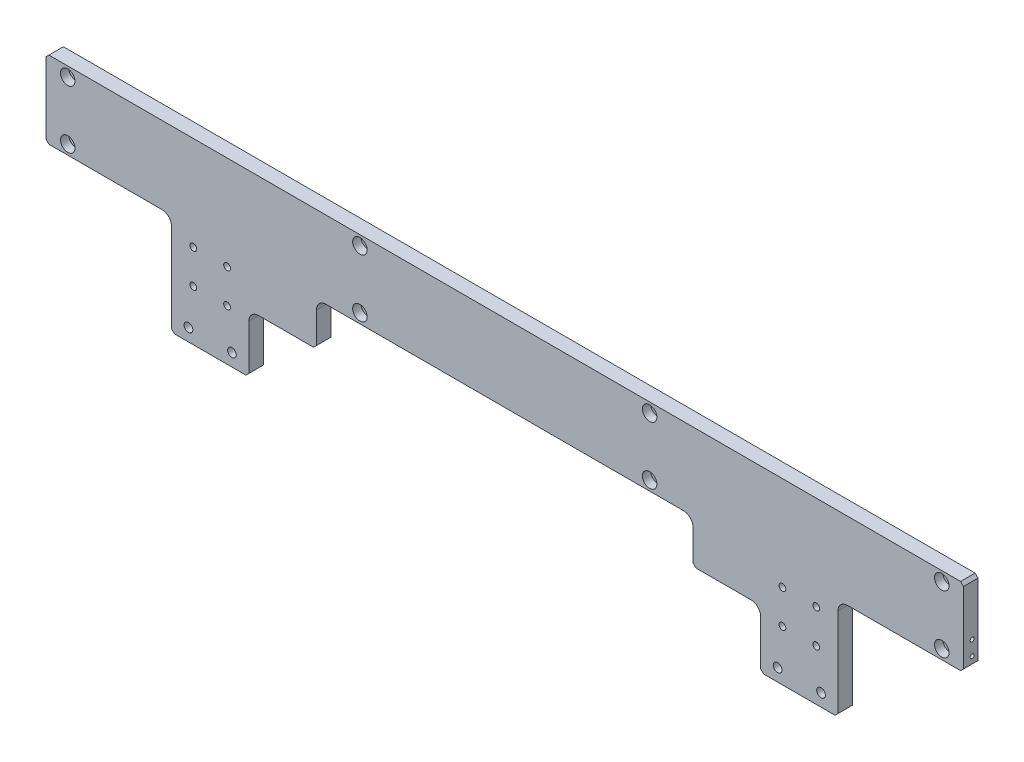
SolidWorks part; units mm, degrees
ref_plane "前视基准面" through (0, 0, 0) normal (0, 0, 1) x (1, 0, 0)
ref_plane "上视基准面" through (0, 0, 0) normal (0, 1, 0) x (1, 0, 0)
ref_plane "右视基准面" through (0, 0, 0) normal (1, 0, 0) x (0, 0, -1)
sketch "草图1" plane through (0, 0, 0) normal (0, 0, 1) x (1, 0, 0)
  line L1 (-475, 40) -> (475, 40)
  line L2 (-475, 40) -> (-475, -40)
  line L3 (-475, -40) -> (475, -40)
  line L4 (475, 40) -> (475, -40)
  line L5 (-475, 40) -> (475, -40) construction
  line L6 (-475, -40) -> (475, 40) construction
  point P0 (0, 0)
  dimension "D1" = 950
  dimension "D2" = 80
extrude "凸台-拉伸1" add sketch "草图1" along normal mid plane 15
hole_wizard "M8 六角凹头螺钉的柱形沉头孔1" positions "草图4" profile "草图3" counterbore size "M8" standard "ISO" end condition through all
sketch "草图4" plane through (0, 0, 7.5) normal (0, 0, 1) x (1, 0, 0)
  line L3 (0, 0) -> (0, 119.4543) construction
  line L4 (0, 0) -> (227.7716, 0) construction
  point P0 (452.5, -30)
  point P2 (452.5, 30)
  point P15 (150, -30)
  point P16 (150, 30)
  point P27 (-452.5, 30)
  point P28 (-452.5, -30)
  point P29 (-150, 30)
  point P30 (-150, -30)
  dimension "D2" = 60
  dimension "D3" = 905
  dimension "D5" = 300
  dimension "D4" = 2
sketch "草图3" plane through (452.5, -30, 7.5) normal (1, 0, 0) x (0, -1, 0)
  line L0 (0, 0) -> (0, 15)
  line L1 (0, 15) -> (4.5, 15)
  line L3 (4.5, 15) -> (4.5, 8.6)
  line L4 (4.5, 8.6) -> (7.5, 8.6)
  line L5 (7.5, 8.6) -> (7.5, 0)
  line L7 (7.5, 0) -> (0, 0)
  line L11 (0, -6.35) -> (0, 107.95) construction
  dimension "通孔孔直径" = 9
  dimension "通孔孔深度" = 15
  dimension "柱形沉头孔直径" = 15
  dimension "柱形沉头孔深度" = 8.6
chamfer "倒角1" distance 3 angle 45 4 edges at (475, -40, 0) (475, 40, 0) (-475, 40, 0) (-475, -40, 0)
sketch "草图7" plane through (0, -40, 0) normal (0, -1, 0) x (1, 0, 0)
  line L0 (-472, -7.5) -> (472, -7.5) construction
  line L1 (345, -7.5) -> (195, -7.5)
  line L2 (345, -7.5) -> (345, 7.5)
  line L3 (345, 7.5) -> (195, 7.5)
  line L4 (195, -7.5) -> (195, 7.5)
  line L5 (-472, 7.5) -> (472, 7.5) construction
  line L6 (475, 7.5) -> (475, -7.5) construction
  dimension "D1" = 130
  dimension "D2" = 150
extrude "凸台-拉伸2" add sketch "草图7" along normal blind 105
ref_plane "基准面1" through (0, 0, 0) normal (1, 0, 0) x (0, 0, -1)
mirror "镜向1" about plane through (0, 0, 0) normal (1, 0, 0) of "凸台-拉伸2"
fillet "圆角1" radius 10 4 edges at (-345, -40, 0) (-195, -40, 0)
hole_wizard "M6 六角凹头螺钉的柱形沉头孔1" positions "草图9" profile "草图8" hole size "Ø7.0" standard "GB" end condition through all
sketch "草图9" plane through (0, 0, -7.5) normal (0, 0, -1) x (-1, 0, 0)
  point P0 (-287.5, -92.5)
  point P3 (-287.5, -57.5)
  point P6 (-322.5, -57.5)
  point P9 (-322.5, -92.5)
sketch "草图8" plane through (287.5, -92.5, -7.5) normal (1, 0, 0) x (0, 1, 0)
  line L0 (0, 0) -> (0, 15)
  line L1 (0, 15) -> (3.5, 15)
  line L2 (3.5, 15) -> (3.5, 0)
  line L5 (3.5, 0) -> (0, 0)
  line L11 (0, -6.35) -> (0, 107.95) construction
  dimension "通孔孔直径" = 7
  dimension "通孔孔深度" = 15
hole_wizard "Ø9.0 (9) 直径孔1" positions "草图11" profile "草图10" hole size "Ø9.0" standard "GB" end condition through all
sketch "草图11" plane through (0, 0, -7.5) normal (0, 0, -1) x (-1, 0, 0)
  point P0 (-282.5, -132)
  point P3 (-327.5, -132)
sketch "草图10" plane through (282.5, -132, -7.5) normal (1, 0, 0) x (0, 1, 0)
  line L0 (0, 0) -> (0, 15)
  line L1 (0, 15) -> (4.5, 15)
  line L2 (4.5, 15) -> (4.5, 0)
  line L5 (4.5, 0) -> (0, 0)
  line L11 (0, -6.35) -> (0, 107.95) construction
  dimension "通孔孔直径" = 9
  dimension "通孔孔深度" = 15
mirror "镜向2" about plane through (0, 0, 0) normal (1, 0, 0) of "Ø9.0 (9) 直径孔1", "M6 六角凹头螺钉的柱形沉头孔1"
hole_wizard "M5 螺纹孔1" positions "草图13" profile "草图14" tap size "M5" standard "ISO"
sketch "草图13" plane through (-475, 0, 0) normal (-1, 0, 0) x (0, 0, 1)
  point P0 (-1.5, -30)
  point P3 (-1.5, -15)
sketch "草图14" plane through (-475, -30, -1.5) normal (0, 1, 0) x (0, 0, 1)
  line L0 (0, 0) -> (0, 13.6618)
  line L1 (0, 13.6618) -> (2.1, 12.4)
  line L2 (2.1, 12.4) -> (2.1, 0)
  line L5 (2.1, 0) -> (0, 0)
  line L10 (0, 13.6618) -> (-2.1, 12.4) construction
  line L11 (0, -6.35) -> (0, 107.95) construction
  dimension "螺纹孔钻头直径" = 4.2
  dimension "螺纹孔钻头深度" = 12.4
  dimension "导头角度" = 118
cosmetic thread "孔螺蚊线1" parameters "D1"=10, "D2"=5
cosmetic thread "孔螺蚊线2" parameters "D1"=10, "D2"=5
hole_wizard "M5 螺纹孔2" positions "草图16" profile "草图15" tap size "M5" standard "ISO"
sketch "草图16" plane through (475, 0, 0) normal (1, 0, 0) x (0, 0, -1)
  point P0 (1.5, -15)
  point P3 (1.5, -30)
sketch "草图15" plane through (475, -15, -1.5) normal (0, 1, 0) x (0, 0, -1)
  line L0 (0, 0) -> (0, 13.6618)
  line L1 (0, 13.6618) -> (2.1, 12.4)
  line L2 (2.1, 12.4) -> (2.1, 0)
  line L5 (2.1, 0) -> (0, 0)
  line L10 (0, 13.6618) -> (-2.1, 12.4) construction
  line L11 (0, -6.35) -> (0, 107.95) construction
  dimension "螺纹孔钻头直径" = 4.2
  dimension "螺纹孔钻头深度" = 12.4
  dimension "导头角度" = 118
cosmetic thread "孔螺蚊线3" parameters "D1"=10, "D2"=5
cosmetic thread "孔螺蚊线4" parameters "D1"=10, "D2"=5
sketch "草图17" plane through (0, 0, -7.5) normal (0, 0, -1) x (-1, 0, 0)
  line L1 (-195, -145) -> (-265, -145)
  line L2 (-195, -145) -> (-195, -85)
  line L3 (-195, -85) -> (-265, -85)
  line L4 (-265, -145) -> (-265, -85)
  circle A0 centre (-282.5, -132) radius 4.5 construction
  dimension "D1" = 17.5
  dimension "D2" = 60
extrude "切除-拉伸1" cut sketch "草图17" against normal through all
mirror "镜向3" about plane through (0, 0, 0) normal (1, 0, 0) of "切除-拉伸1"
fillet "圆角2" radius 10 2 edges at (-265, -85, 0) (265, -85, 0)
chamfer "倒角3" distance 3 angle 45 6 edges at (-345, -145, 0) (-265, -145, 0) (-195, -85, 0) (195, -85, 0) (265, -145, 0) (345, -145, 0)
